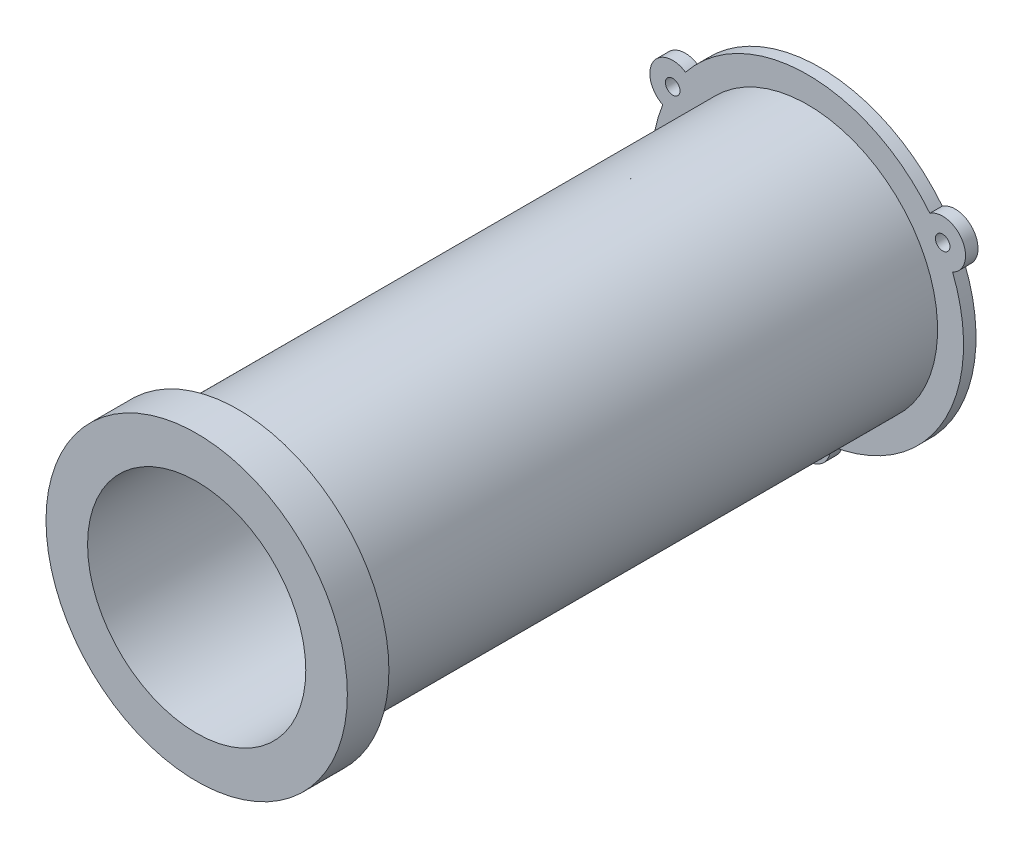
SolidWorks part; units mm, degrees
ref_plane "前视基准面" through (0, 0, 0) normal (0, 0, 1) x (1, 0, 0)
ref_plane "上视基准面" through (0, 0, 0) normal (0, 1, 0) x (1, 0, 0)
ref_plane "右视基准面" through (0, 0, 0) normal (1, 0, 0) x (0, 0, -1)
sketch "草图1" plane through (0, 0, 0) normal (0, 0, 1) x (1, 0, 0)
  circle A0 centre (0, 0) radius 62.5
  circle A1 centre (0, 0) radius 52.5
  dimension "D1" = 105
  dimension "D2" = 125
extrude "凸台-拉伸1" add sketch "草图1" along normal blind 284
sketch "草图2" plane through (0, 0, 284) normal (0, 0, 1) x (1, 0, 0)
  circle A0 centre (0, 0) radius 52.5
  circle A1 centre (0, 0) radius 72.5
  dimension "D1" = 145
  dimension "D2" = 105
extrude "凸台-拉伸2" add sketch "草图2" along normal mid plane 20
sketch "草图3" plane through (0, 0, 0) normal (0, 0, -1) x (-1, 0, 0)
  arc A0 (10.9704, -74.1933) -> (69.7385, 27.596) centre (0, 0) ccw
  circle A1 centre (0, 0) radius 52.5
  circle A2 centre (0, -75) radius 3.5
  arc A3 (-10.9704, -74.1933) -> (10.9704, -74.1933) centre (0, -75) ccw
  arc A4 (-58.7681, 46.5973) -> (-69.7385, 27.596) centre (-64.9519, 37.5) ccw
  circle A5 centre (-64.9519, 37.5) radius 3.5
  arc A6 (69.7385, 27.596) -> (58.7681, 46.5973) centre (64.9519, 37.5) ccw
  circle A7 centre (64.9519, 37.5) radius 3.5
  arc A8 (58.7681, 46.5973) -> (-58.7681, 46.5973) centre (0, 0) ccw
  arc A9 (-69.7385, 27.596) -> (-10.9704, -74.1933) centre (0, 0) ccw
  point P6 (0, 0)
  point P18 (0, 0)
  dimension "D1" = 150
  dimension "D2" = 7
  dimension "D3" = 22
  dimension "D5" = 105
  dimension "D4" = 3
extrude "凸台-拉伸3" add sketch "草图3" along normal blind 6
